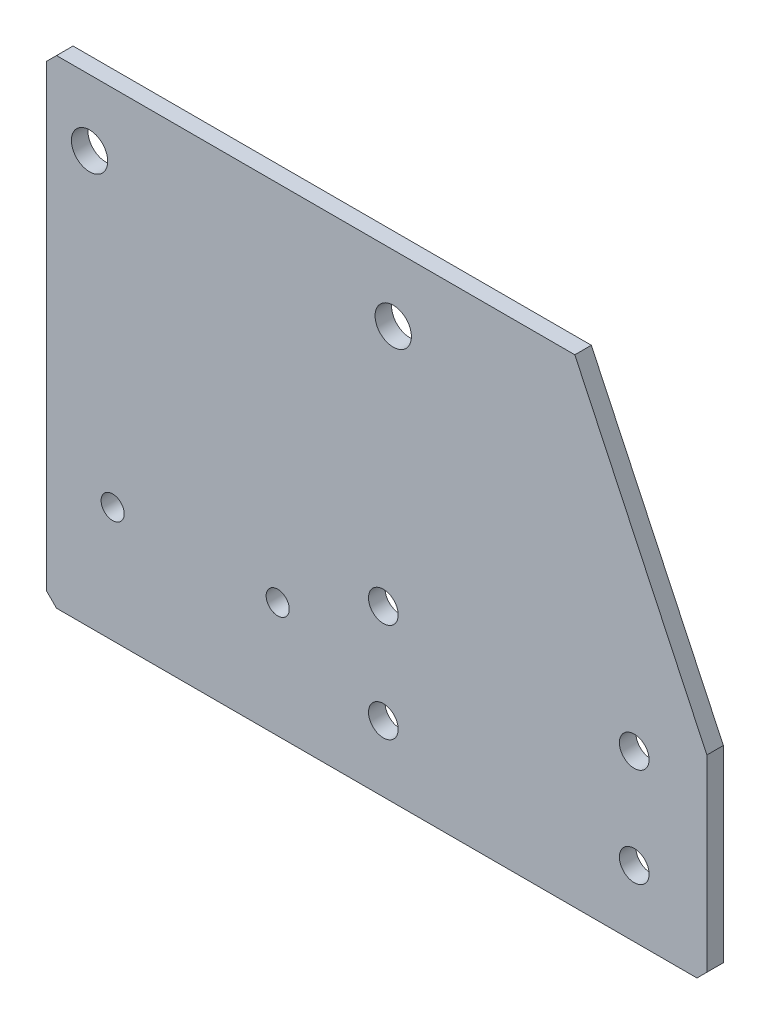
from build123d import *

# Parameters (mm, degrees)
SKETCH_1_R      = 4.5
SKETCH_1_R_2    = 3.5
SKETCH_1_R_3    = 5.5
EXTRUDE_1_DEPTH = 5


with BuildPart() as part:
    # 草图1 → 凸台-拉伸1 (new body)
    with BuildSketch(Plane.XY.offset(2.5)):
        Polygon((-97, -72.5), (97, -72.5), (100, -69.5), (100, -12.5), (60, 72.5), (-97, 72.5), (-100, 69.5), (-100, -69.5), align=None)
        with Locations(Location((2, -22.5, 0), (0, 0, 180))):
            Circle(SKETCH_1_R, mode=Mode.SUBTRACT)
        with Locations(Location((-30, -37.5, 0), (0, 0, 180))):
            Circle(SKETCH_1_R_2, mode=Mode.SUBTRACT)
        with Locations(Location((-80, -37.5, 0), (0, 0, 180))):
            Circle(SKETCH_1_R_2, mode=Mode.SUBTRACT)
        with Locations(Location((5, 52.5, 0), (0, 0, 180))):
            Circle(SKETCH_1_R_3, mode=Mode.SUBTRACT)
        with Locations(Location((78, -52.5, 0), (0, 0, 180))):
            Circle(SKETCH_1_R, mode=Mode.SUBTRACT)
        with Locations(Location((2, -52.5, 0), (0, 0, 180))):
            Circle(SKETCH_1_R, mode=Mode.SUBTRACT)
        with Locations(Location((78, -22.5, 0), (0, 0, 180))):
            Circle(SKETCH_1_R, mode=Mode.SUBTRACT)
        with Locations(Location((-87, 52.5, 0), (0, 0, 180))):
            Circle(SKETCH_1_R_3, mode=Mode.SUBTRACT)
    extrude(amount=-EXTRUDE_1_DEPTH)


solid = part.part
